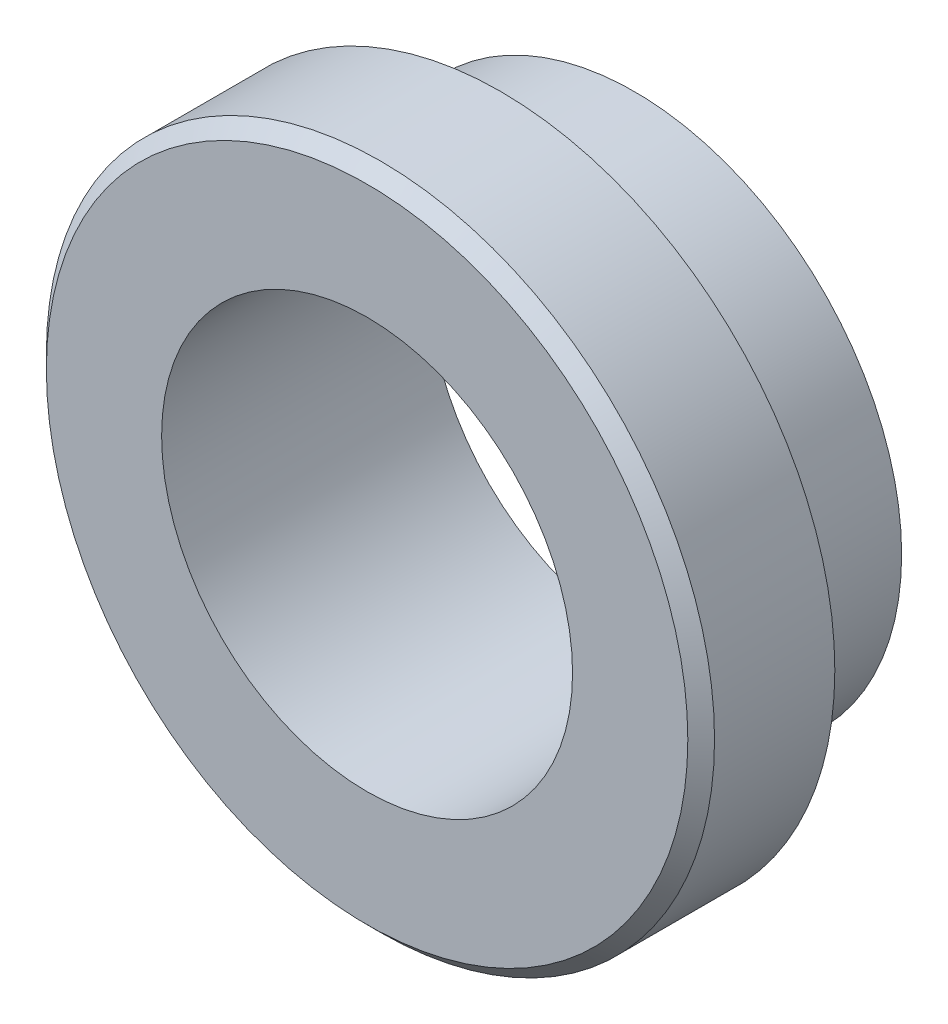
SolidWorks part; units mm, degrees
material "45#调质"
ref_plane "Front Plane" through (0, 0, 0) normal (0, 0, 1) x (1, 0, 0)
ref_plane "Top Plane" through (0, 0, 0) normal (0, 1, 0) x (1, 0, 0)
ref_plane "Right Plane" through (0, 0, 0) normal (1, 0, 0) x (0, 0, -1)
sketch "Sketch1" plane through (0, 0, 0) normal (1, 0, 0) x (0, 0, -1)
  line L0 (0, 0) -> (0, 20)
  line L1 (0, 20) -> (-10, 20)
  line L2 (-10, 20) -> (-10, 25)
  line L3 (-10, 25) -> (-20, 25)
  line L4 (-20, 25) -> (-20, 0)
  line L5 (-20, 0) -> (0, 0)
  dimension "D1" = 20
  dimension "D2" = 5
  dimension "D3" = 10
  dimension "D4" = 10
revolve "Revolve1" add sketch "Sketch1" angle 360 about L5
hole_wizard "G1 Tapped Hole1" positions "Sketch2" profile "Sketch3" tap size "G1" standard "GB" end condition through all
sketch "Sketch2" plane through (0, 0, 20) normal (0, 0, 1) x (1, 0, 0)
  point P0 (0, 0)
sketch "Sketch3" plane through (0, 0, 20) normal (1, 0, 0) x (0, -1, 0)
  line L0 (0, 0) -> (0, 20)
  line L1 (0, 20) -> (15.375, 20)
  line L2 (15.375, 20) -> (15.375, 0)
  line L5 (15.375, 0) -> (0, 0)
  line L11 (0, -6.35) -> (0, 107.95) construction
  dimension "通孔螺纹孔钻头直径" = 30.75
  dimension "通孔螺纹孔钻头深度" = 20
cosmetic thread "Cosmetic thread1"
chamfer "Chamfer1" distance 1 angle 45 1 edges at (25, 0, 20)
